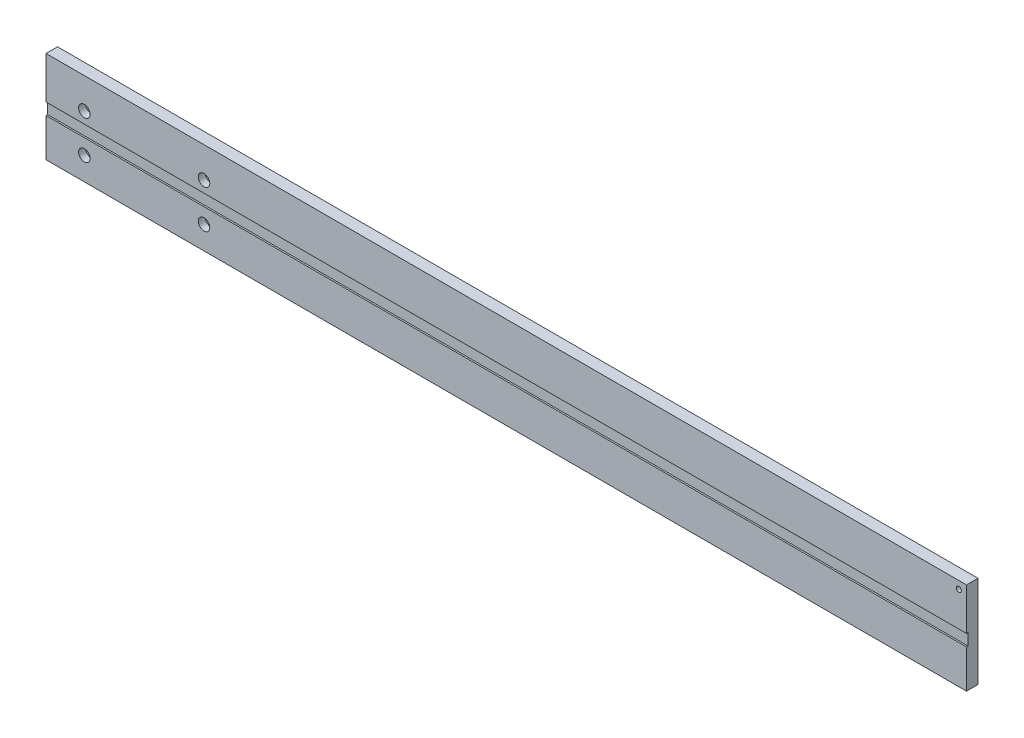
SolidWorks part; units mm, degrees
ref_plane "前视基准面" through (0, 0, 0) normal (0, 0, 1) x (1, 0, 0)
ref_plane "上视基准面" through (0, 0, 0) normal (0, 1, 0) x (1, 0, 0)
ref_plane "右视基准面" through (0, 0, 0) normal (1, 0, 0) x (0, 0, -1)
sketch "草图1" plane through (0, 0, 0) normal (0, 0, 1) x (1, 0, 0)
  line L1 (-600, 60) -> (600, 60)
  line L2 (-600, 60) -> (-600, -60)
  line L3 (-600, -60) -> (600, -60)
  line L4 (600, 60) -> (600, -60)
  line L5 (-600, 60) -> (600, -60) construction
  line L6 (-600, -60) -> (600, 60) construction
  point P0 (0, 0)
  dimension "D1" = 1200
  dimension "D2" = 120
extrude "凸台-拉伸1" add sketch "草图1" along normal mid plane 15
hole_wizard "打孔尺寸(%根据)内六角圆柱头螺钉的类型3" positions "3D草图1" profile "草图3" counterbore size "M6" standard "GB" end condition through all
sketch3d "3D草图1"
  line L0 (600, 60, -7.5) -> (-600, 60, -7.5) construction
  line L1 (600, -60, -7.5) -> (600, 60, -7.5) construction
  point P0 (590, 50, -7.5)
  dimension "D1" = 10
  dimension "D2" = 10
sketch "草图3" plane through (590, 50, -7.5) normal (1, 0, 0) x (0, 1, 0)
  line L0 (0, 0) -> (0, 15)
  line L1 (0, 15) -> (3.3, 15)
  line L3 (3.3, 15) -> (3.3, 6.8)
  line L4 (3.3, 6.8) -> (5.5, 6.8)
  line L5 (5.5, 6.8) -> (5.5, 0)
  line L7 (5.5, 0) -> (0, 0)
  line L11 (0, -6.35) -> (0, 107.95) construction
  dimension "通孔孔直径" = 6.6
  dimension "通孔孔深度" = 15
  dimension "柱形沉头孔直径" = 11
  dimension "柱形沉头孔深度" = 6.8
hole_wizard "打孔尺寸(%根据)内六角圆柱头螺钉的类型3" positions "3D草图3" profile "草图6" counterbore size "M8" standard "GB" end condition through all
sketch3d "3D草图3"
  line L0 (600, 60, 7.5) -> (-600, 60, 7.5) construction
  line L1 (-600, 60, 7.5) -> (-600, -60, 7.5) construction
  line L2 (-600, -60, 7.5) -> (600, -60, 7.5) construction
  point P0 (-550, 20, 7.5)
  point P2 (-394, 20, 7.5)
  point P4 (-394, -30, 7.5)
  point P6 (-550, -30, 7.5)
  dimension "D1" = 40
  dimension "D2" = 50
  dimension "D3" = 50
  dimension "D4" = 30
  dimension "D5" = 206
  dimension "D6" = 40
  dimension "D7" = 30
  dimension "D8" = 206
sketch "草图6" plane through (-550, 20, 7.5) normal (1, 0, 0) x (0, -1, 0)
  line L0 (0, 0) -> (0, 15)
  line L1 (0, 15) -> (4.5, 15)
  line L3 (4.5, 15) -> (4.5, 9)
  line L4 (4.5, 9) -> (7.5, 9)
  line L5 (7.5, 9) -> (7.5, 0)
  line L7 (7.5, 0) -> (0, 0)
  line L11 (0, -6.35) -> (0, 107.95) construction
  dimension "通孔孔直径" = 9
  dimension "通孔孔深度" = 15
  dimension "柱形沉头孔直径" = 15
  dimension "柱形沉头孔深度" = 9
sketch "草图7" plane through (600, 0, 0) normal (1, 0, 0) x (0, 0, -1)
  line L0 (-7.5, -60) -> (-7.5, 60) construction
  line L1 (-7.5, 5.2) -> (-5.5, 5.2)
  line L2 (-7.5, 5.2) -> (-7.5, -10)
  line L3 (-7.5, -10) -> (-5.5, -10)
  line L4 (-5.5, 5.2) -> (-5.5, -10)
  line L6 (-7.5, -60) -> (7.5, -60) construction
  dimension "D1" = 15.2
  dimension "D2" = 2
  dimension "D3" = 50
extrude "切除-拉伸1" cut sketch "草图7" against normal through all
